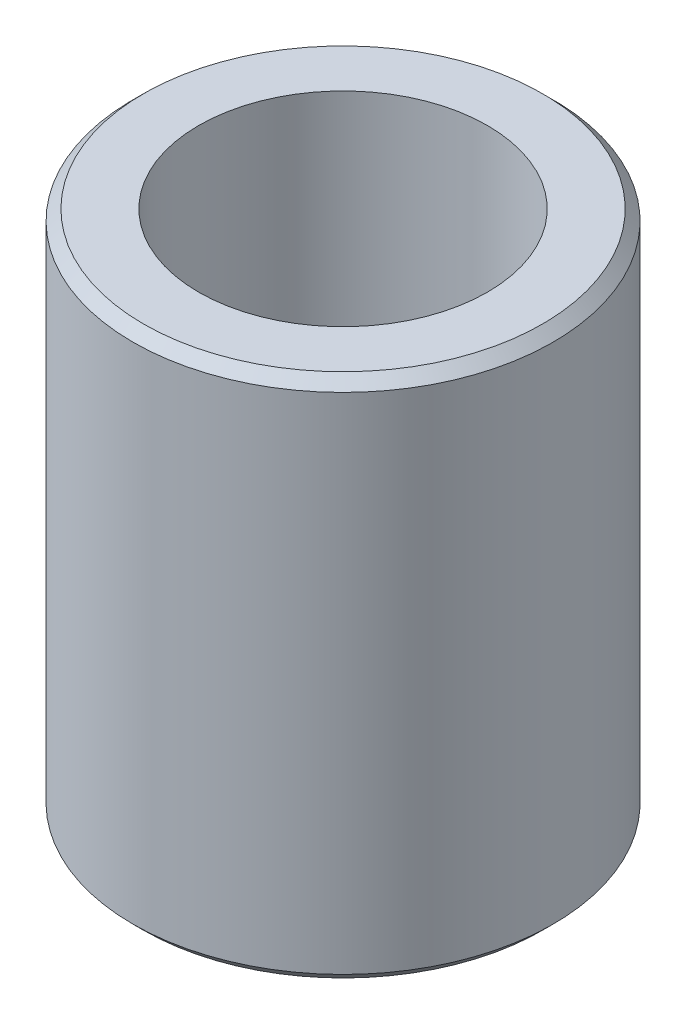
SolidWorks part; units mm, degrees
ref_plane "Front Plane" through (0, 0, 0) normal (0, 0, 1) x (1, 0, 0)
ref_plane "Top Plane" through (0, 0, 0) normal (0, 1, 0) x (1, 0, 0)
ref_plane "Right Plane" through (0, 0, 0) normal (1, 0, 0) x (0, 0, -1)
sketch "Sketch1" plane through (0, 0, 0) normal (0, 1, 0) x (1, 0, 0)
  circle A0 centre (0, 0) radius 2.75
  circle A1 centre (0, 0) radius 4
  dimension "D1" = 8
  dimension "D2" = 5.5
extrude "Boss-Extrude1" add sketch "Sketch1" along normal blind 10
chamfer "Chamfer1" distance 0.2 angle 45 2 edges at (0, 0, 4) (0, 10, 4)
